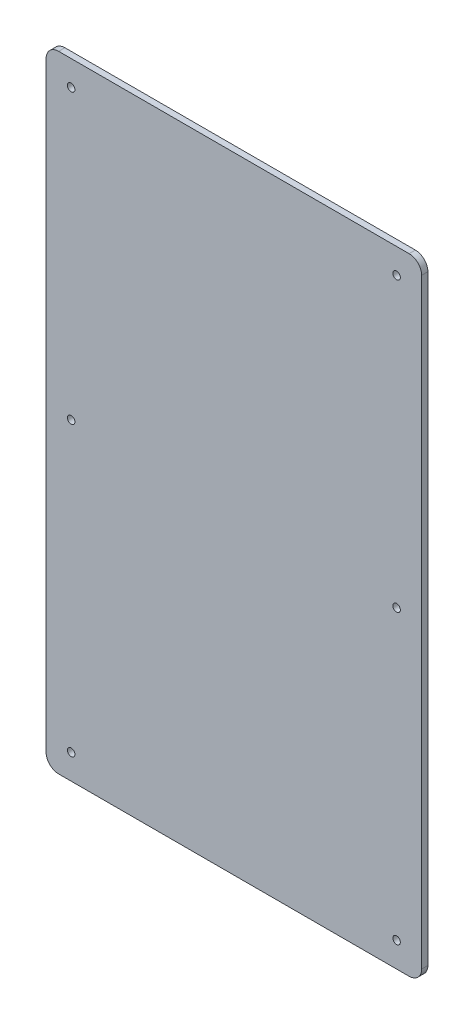
SolidWorks part; units mm, degrees
material "PMMA（透明）"
ref_plane "前视基准面" through (0, 0, 0) normal (0, 0, 1) x (1, 0, 0)
ref_plane "上视基准面" through (0, 0, 0) normal (0, 1, 0) x (1, 0, 0)
ref_plane "右视基准面" through (0, 0, 0) normal (1, 0, 0) x (0, 0, -1)
sketch "草图1" plane through (0, 0, 0) normal (0, 0, 1) x (1, 0, 0)
  line L1 (-150, -250) -> (150, -250)
  line L2 (-150, -250) -> (-150, 250)
  line L3 (-150, 250) -> (150, 250)
  line L4 (150, -250) -> (150, 250)
  line L5 (-150, -250) -> (150, 250) construction
  line L6 (-150, 250) -> (150, -250) construction
  point P0 (0, 0)
  dimension "D1" = 300
  dimension "D2" = 500
extrude "凸台-拉伸1" add sketch "草图1" along normal blind 5
hole_wizard "Ø6.0 (6) 直径孔1" positions "草图2" profile "草图3" hole size "Ø6.0" standard "ISO"
sketch "草图2" plane through (0, 0, 5) normal (0, 0, 1) x (1, 0, 0)
  line L0 (-150, 0) -> (150, 0) construction
  line L1 (-150, 250) -> (-150, -250) construction
  line L2 (150, -250) -> (150, 250) construction
  line L4 (0, 250) -> (0, -250) construction
  line L5 (150, 250) -> (-150, 250) construction
  line L6 (-150, -250) -> (150, -250) construction
  point P0 (-130, 230)
  point P2 (130, 230)
  point P21 (130, -230)
  point P22 (-130, -230)
  point P23 (-130, 0)
  point P27 (130, 0)
  dimension "D1" = 20
  dimension "D2" = 20
sketch "草图3" plane through (-130, 230, 5) normal (1, 0, 0) x (0, -1, 0)
  line L0 (0, 0) -> (0, 29.5526)
  line L1 (0, 29.5526) -> (3, 27.75)
  line L2 (3, 27.75) -> (3, 0)
  line L5 (3, 0) -> (0, 0)
  line L10 (0, 29.5526) -> (-3, 27.75) construction
  line L11 (0, -6.35) -> (0, 107.95) construction
  dimension "孔直径" = 6
  dimension "孔深度" = 27.75
  dimension "导头角度" = 118
fillet "圆角1" radius 10 4 edges at (-150, -250, 2.5) (150, -250, 2.5) (150, 250, 2.5) (-150, 250, 2.5)
